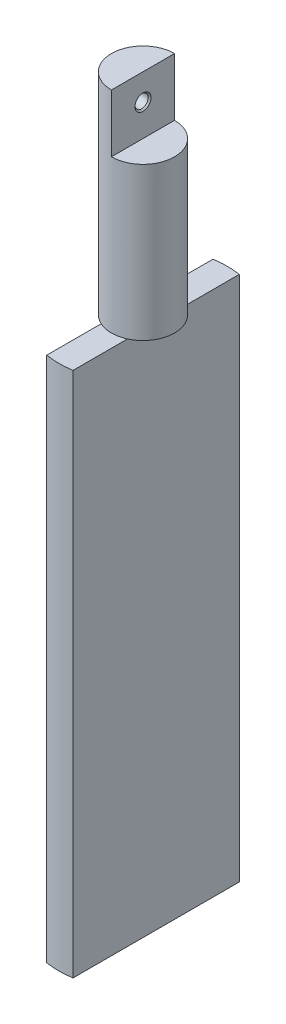
SolidWorks part; units mm, degrees
ref_plane "Front Plane" through (0, 0, 0) normal (0, 0, 1) x (1, 0, 0)
ref_plane "Top Plane" through (0, 0, 0) normal (0, 1, 0) x (1, 0, 0)
ref_plane "Right Plane" through (0, 0, 0) normal (1, 0, 0) x (0, 0, -1)
other "Configuration Table"
sketch "Sketch1" plane through (0, 0, 0) normal (0, 1, 0) x (1, 0, 0)
  circle A0 centre (0, 0) radius 6
  dimension "D1" = 12
extrude "Boss-Extrude1" add sketch "Sketch1" along normal blind 40
sketch "Sketch2" plane through (0, 0, 0) normal (0, 0, 1) x (1, 0, 0)
  line L0 (6, 40) -> (-6, 40) construction
  line L1 (0, 40) -> (18.4702, 40)
  line L2 (0, 40) -> (0, 29)
  line L3 (0, 29) -> (18.4702, 29)
  line L4 (18.4702, 40) -> (18.4702, 29)
  dimension "D1" = 11
extrude "Cut-Extrude1" cut sketch "Sketch2" against normal through all both and the other way through all
sketch "Sketch3" plane through (0, 0, 0) normal (1, 0, 0) x (0, 0, -1)
  line L0 (0, 0) -> (0, 35) construction
  line L1 (6, 29) -> (-6, 29) construction
  point P1 (0, 35)
  point P7 (0, 35)
  dimension "D1" = 6
hole_wizard "M3 Tapped Hole2" positions "Sketch3" profile "Sketch4" tap size "M3" standard "GB" end condition through all
cosmetic thread "Hole cosmetic thread1" parameters "D2"=3
sketch "Sketch4" plane through (0, 35, 0) normal (0, 1, 0) x (0, 0, -1)
  line L0 (0, 0) -> (0, 6)
  line L1 (0, 6) -> (1.25, 6)
  line L2 (1.25, 6) -> (1.25, 0.275)
  line L3 (1.25, 0.275) -> (1.525, 0)
  line L5 (1.525, 0) -> (0, 0)
  line L6 (-1.25, 0.275) -> (-1.525, 0) construction
  line L11 (0, -6.35) -> (0, 107.95) construction
  dimension "通孔螺纹孔钻头直径" = 2.5
  dimension "通孔螺纹孔钻头深度" = 6
  dimension "近端锥形沉头孔直径" = 3.05
  dimension "近端锥形沉头孔角度" = 90
sketch "Sketch5" plane through (0, 0, 0) normal (0, -1, 0) x (1, 0, 0)
  circle A0 centre (0, 0) radius 16
  dimension "D1" = 32
extrude "Boss-Extrude2" add sketch "Sketch5" along normal blind 100
sketch "Sketch11" plane through (0, -100, 0) normal (0, -1, 0) x (1, 0, 0)
  line L1 (-2.5, 20.2126) -> (2.5, 20.2126)
  line L2 (-2.5, 20.2126) -> (-2.5, -20.2126)
  line L3 (-2.5, -20.2126) -> (2.5, -20.2126)
  line L4 (2.5, 20.2126) -> (2.5, -20.2126)
  line L5 (-2.5, 20.2126) -> (2.5, -20.2126) construction
  line L6 (-2.5, -20.2126) -> (2.5, 20.2126) construction
  point P0 (0, 0)
  dimension "D1" = 5
extrude "Cut-Extrude2" cut sketch "Sketch11" against normal up to surface (100 mm away) and the other way through all flip side to cut up to face at (0, 0, 6)
